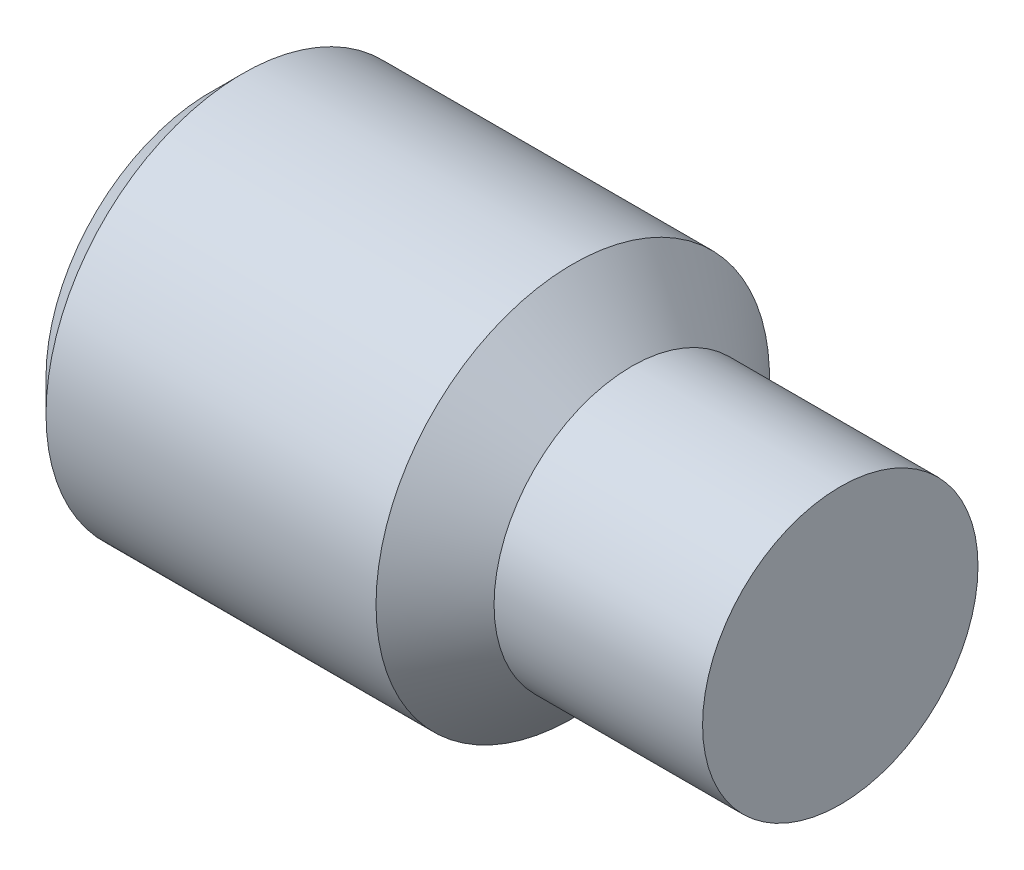
from build123d import *

# Parameters (mm, degrees)
HEXAGONSOCKET_DEPTH = 4


with BuildPart() as part:
    # Sketch1 → Base (revolve)
    with BuildSketch(Plane.XY, mode=Mode.PRIVATE) as base_sk:
        Polygon((0, 0), (16, 0), (16, 3.5), (10.7, 3.5), (9.2, 5), (0.812, 5), (0, 4.188), align=None)
    revolve(base_sk.sketch.rotate(Axis((-1.968820569, 0, 0), (1, 0, 0)), 90), axis=Axis((-1.968820569, 0, 0), (1, 0, 0)))

    # Sketch2 → HexagonSocket (cut)
    with BuildSketch(Plane(origin=(0, -1.128463942, -0.35035393), x_dir=(0, 0, 1), z_dir=(-1, 0, 0))):
        Polygon((3.237105276, 1.128463942), (1.793729603, 3.628463942), (-1.093021743, 3.628463942), (-2.536397416, 1.128463942), (-1.093021743, -1.371536058), (1.793729603, -1.371536058), align=None)
    extrude(amount=-HEXAGONSOCKET_DEPTH, mode=Mode.SUBTRACT)

    # Sketch3 → Cut-Revolve1 (revolve, cut)
    with BuildSketch(Plane.XY, mode=Mode.PRIVATE) as cut_revolve1_sk:
        Polygon((4, 2.5), (4, 0), (4.8, 0), align=None)
    revolve(cut_revolve1_sk.sketch.rotate(Axis((-0.330994676, 0, 0), (1, 0, 0)), 90), axis=Axis((-0.330994676, 0, 0), (1, 0, 0)), mode=Mode.SUBTRACT)


solid = part.part
